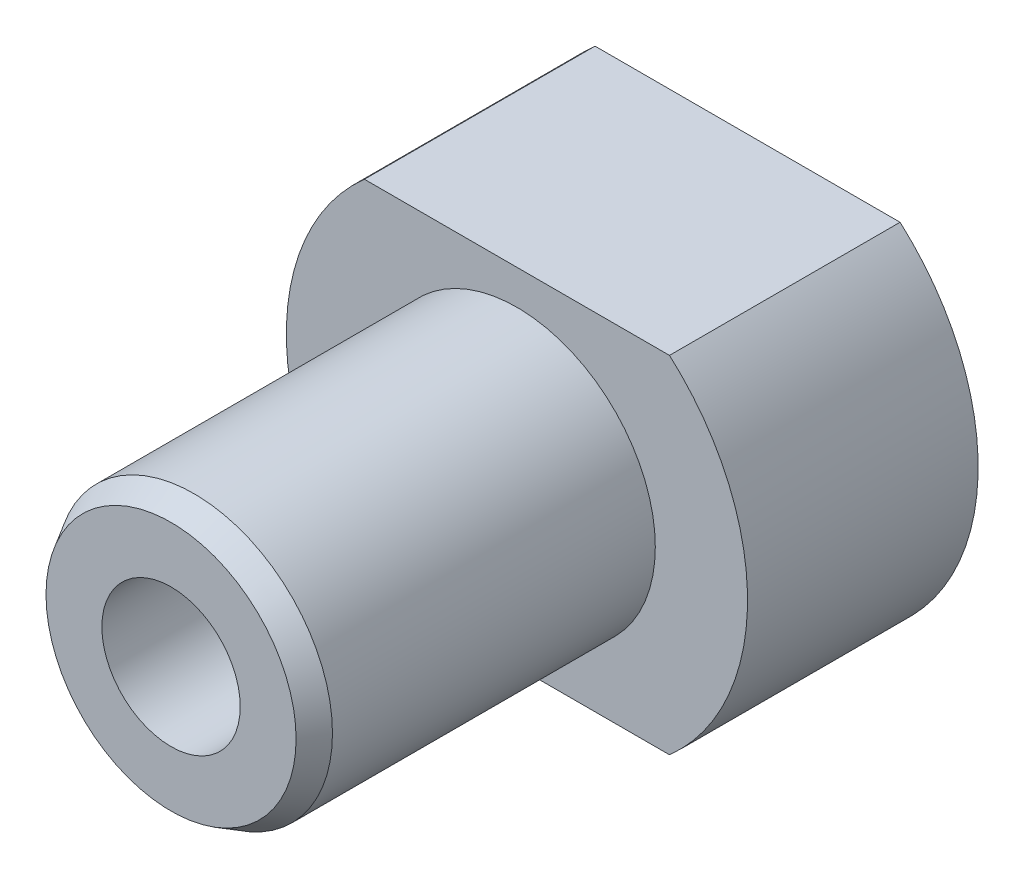
from build123d import *
from build123d.topology import SkipClean

# Parameters (mm, degrees)
SKETCH1_R           = 6
SKETCH1_R_2         = 3
BOSS_EXTRUDE1_DEPTH = 15
CHAMFER1_SIZE       = 1
CHAMFER1_SIZE2      = 0.577350269
BOSS_EXTRUDE2_START = 10
SKETCH2_R           = 10
SKETCH2_R_2         = 3
BOSS_EXTRUDE2_DEPTH = 10
CUT_EXTRUDE1_DEPTH  = 29.722813233


with BuildPart() as part:
    # Sketch1 → Boss-Extrude1 (new body)
    with BuildSketch(Plane.XY):
        Circle(SKETCH1_R)
        Circle(SKETCH1_R_2, mode=Mode.SUBTRACT)
    extrude(amount=BOSS_EXTRUDE1_DEPTH)

    # Chamfer1
    chamfer1_edges = [part.edges().sort_by_distance(p)[0] for p in [
        (-6, 0, 15),
    ]]
    chamfer1_side = [part.faces().sort_by_distance(p)[0] for p in [
        (-6, 0, 7.5),
    ]]
    chamfer(chamfer1_edges, length=CHAMFER1_SIZE, length2=CHAMFER1_SIZE2, reference=chamfer1_side[0])

    # Sketch2 → Boss-Extrude2 (add)
    with SkipClean():  # the faces are left unmerged after this step: merging them gives an invalid solid
        with BuildSketch(Plane(origin=(0, 0, 0), x_dir=(-1, 0, 0), z_dir=(0, 0, -1)).offset(BOSS_EXTRUDE2_START)):
            Circle(SKETCH2_R)
            Circle(SKETCH2_R_2, mode=Mode.SUBTRACT)
        extrude(amount=-BOSS_EXTRUDE2_DEPTH)

    # Sketch3 → Cut-Extrude1 (cut, through all)
    with SkipClean():  # the faces are left unmerged after this step: merging them gives an invalid solid
        with BuildSketch(Plane(origin=(0, 0, -10), x_dir=(-1, 0, 0), z_dir=(0, 0, -1))):
            Polygon((-12.432586445, 7.5), (-12.432586445, 16.991345965), (16.514398983, 13.775765777), (12.432586445, 7.5), align=None)
            Polygon((-12.432586445, -7.5), (12.432586445, -7.5), (9.879584392, -18.980106847), (-12.432586445, -18.242292142), align=None)
        extrude(amount=-CUT_EXTRUDE1_DEPTH, mode=Mode.SUBTRACT)


solid = part.part
